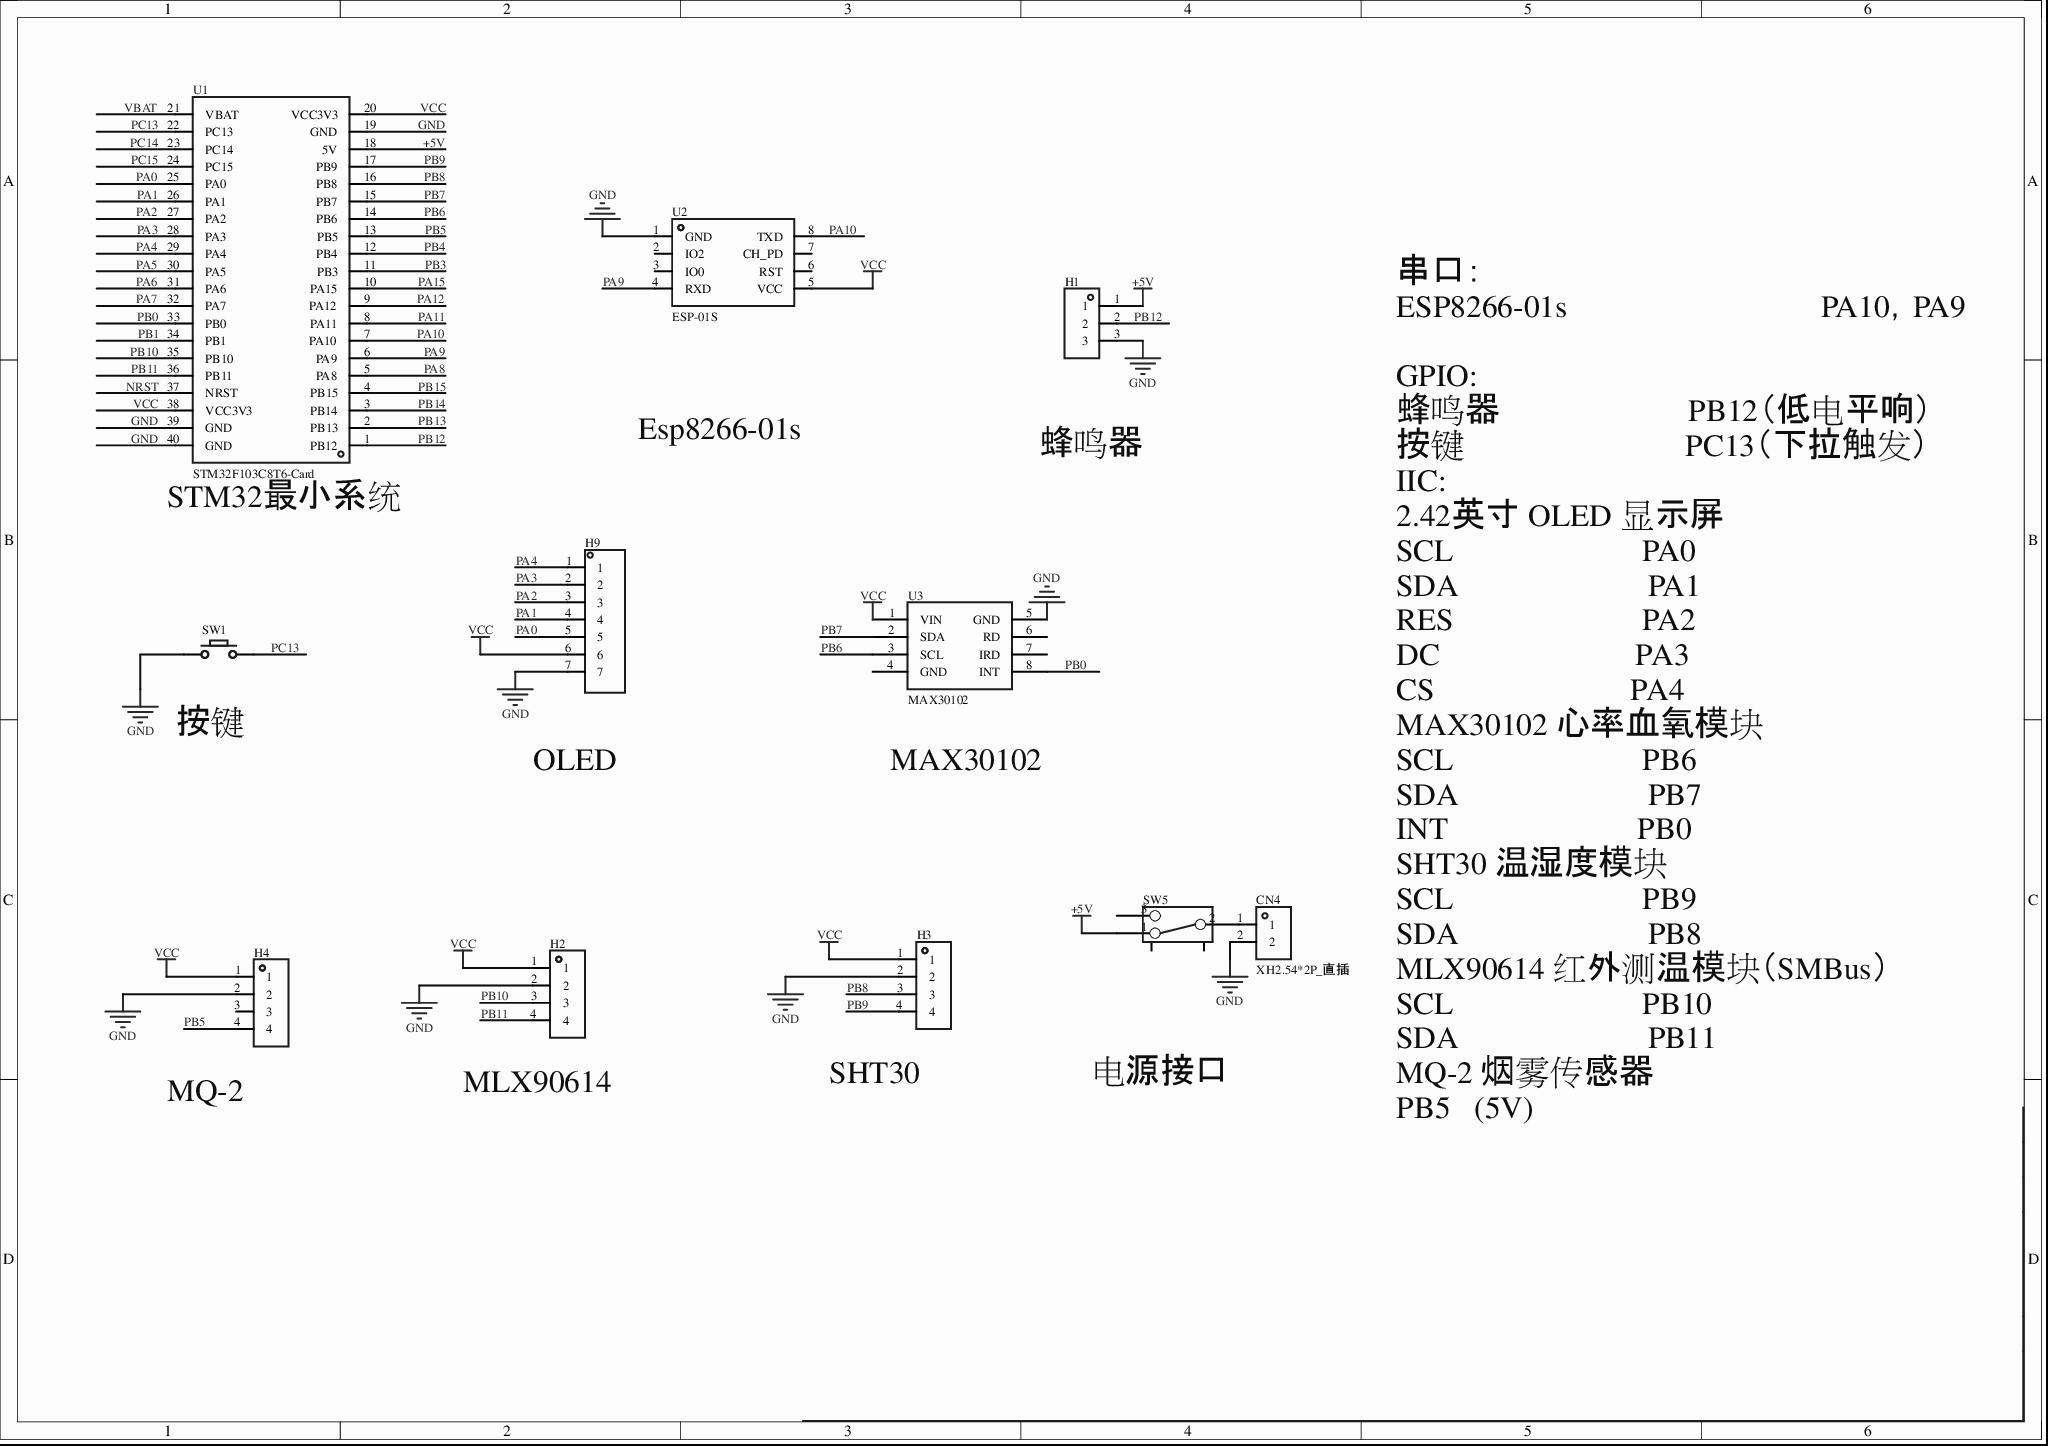
[diagram p0: MISC52061-3.schdoc]
# Altium project MISC52061-2.PrjPcb
1 sheet, 11 parts. Net scope: global (net labels, ports and power ports of the same name join across sheets).
Board file: MISC52061.pcbdoc

## Sheet MISC52061-3.schdoc
size 297 x 209 mm; Version: V1.0; @Project Name: MISC52061; @Page Count: 1; @Update Date: 2026-05-04; @Create Date: 2026-05-04; @Schematic Name: MISC52061; @Page No: 1; @Create Time: 23:22:16; @Update Time: 17:32:40; @Board Name: MISC52061

### Parts
CN4  XH2.54*2P_直插  [CONN-TH_2P-P2.50-XH2.54-2P]
H1  (no value)  [HDR-TH_3P-P2.54-V-F]
H2  (no value)  [HDR-TH_4P-P2.54-V-F]
H3  (no value)  [HDR-TH_4P-P2.54-V-F]
H4  (no value)  [HDR-TH_4P-P2.54-V-F]
H9  (no value)  [HDR-TH_7P-P2.54-V-F]
SW1  (no value)  [Key_TH_3.5x6x4.3]
SW5  (no value)  [拨动开关]
U1  STM32F103C8T6-Card  [CONN-TH_L53.3-W22.9_STM32F103C8T6-CARD]
U2  ESP-01S  [WIFIM-TH_ESP-01S]
U3  MAX30102  [MAX30102]

### Nets
+5V: H1.1 SW5.1 U1.18(5V)
GND: CN4.2 H1.3 H2.2 H3.2 H4.2 H9.7 SW1.A U1.19(GND) U1.39(GND) U1.40(GND) U2.1(GND) U3.5(GND)
VCC: H2.1 H3.1 H4.1 H9.6 U1.20(VCC3V3) U1.38(VCC3V3) U2.5(VCC) U3.1(VIN)
NRST: U1.37(NRST)
PA0: H9.5 U1.25(PA0)
PA1: H9.4 U1.26(PA1)
PA2: H9.3 U1.27(PA2)
PA3: H9.2 U1.28(PA3)
PA4: H9.1 U1.29(PA4)
PA5: U1.30(PA5)
PA6: U1.31(PA6)
PA7: U1.32(PA7)
PA8: U1.5(PA8)
PA9: U1.6(PA9) U2.4(RXD)
PA10: U1.7(PA10) U2.8(TXD)
PA11: U1.8(PA11)
PA12: U1.9(PA12)
PA15: U1.10(PA15)
PB0: U1.33(PB0) U3.8(INT)
PB1: U1.34(PB1)
PB3: U1.11(PB3)
PB4: U1.12(PB4)
PB5: H4.4 U1.13(PB5)
PB6: U1.14(PB6) U3.3(SCL)
PB7: U1.15(PB7) U3.2(SDA)
PB8: H3.3 U1.16(PB8)
PB9: H3.4 U1.17(PB9)
PB10: H2.3 U1.35(PB10)
PB11: H2.4 U1.36(PB11)
PB12: H1.2 U1.1(PB12)
PB13: U1.2(PB13)
PB14: U1.3(PB14)
PB15: U1.4(PB15)
PC13: SW1.B U1.22(PC13)
PC14: U1.23(PC14)
PC15: U1.24(PC15)
VBAT: U1.21(VBAT)
NetCN4_1: CN4.1 SW5.2

Not connected (* = marked no-connect by the designer): H4 3; SW5 3 4 5; U2 2(IO2)* 3(IO0)* 6(RST)* 7(CH_PD)*; U3 4(GND)* 6(RD)* 7(IRD)*

### Notes on the sheet
- 串口：
  ESP8266-01s  		PA10，PA9 	(串口1）
  GPIO:
  蜂鸣器      PB12（低电平响）
  按键       PC13（下拉触发）
  IIC:
  2.42英寸 OLED 显示屏
  SCL      PA0
  SDA      PA1
  RES      PA2
  DC       PA3
  CS       PA4
  MAX30102 心率血氧模块
  SCL      PB6
  SDA      PB7
  INT      PB0
  SHT30 温湿度模块
  SCL      PB9
  SDA      PB8
  MLX90614 红外测温模块（SMBus）
  SCL      PB10
  SDA      PB11
  MQ-2 烟雾传感器   
  PB5   (5V)
- (near U1) STM32最小系统
- Esp8266-01s
- 蜂鸣器
- (near SW1) 按键
- OLED
- MAX30102
- (near H4) MQ-2
- (near H2) MLX90614
- (near H3) SHT30
- 电源接口

### Library data of the parts
CN4 = XH2.54*2P_直插: 3D Model: 325c595e30db4df8abe76612dd40b0fa0819f05c4eef4c71ace90d822a990e87; 3D Model Transform: 295.275,228.346,0,180,0,0,-0.002,-20.079,-137.795; AddInBom: yes; Device: XH2.54*2P_直插; Symbol: XH2.54*2P_直插; LCSC Part Name: XH2.54*2P_直插; Supplier Part: C9900008615; Manufacturer Part: XH2.54*2P_直插; Supplier Footprint: XH2.54_2P; JLCPCB Part Class: Extended Part; Supplier: LCSC; FootprintName: CONN-TH_2P-P2.50-XH2.54-2P; ConvertToPcb: yes; ModelName: CONN-TH_2P-P2.50-XH2.54-2P
H1 = HDR-F_2.54_1x3P: Symbol: PM254V-11-03-H85; 3D Model: f3b3cc5aae9641bf9e56fc160cef875b; 3D Model Transform: 299.9994,100,0,0,0,0,0,0,-118.11; ConvertToPcb: yes; ModelName: HDR2.54-F-LI-1X3P; Device: HDR-F_2.54_1x3P; Supplier Part: C541850; Supplier Footprint: 插件; FootprintName: HDR-TH_3P-P2.54-V-F; AddInBom: yes
H2 H3 = HDR-F_2.54_1x4P: Symbol: 2.54-1*4P母; 3D Model: d187812051054f85879fcaa51a310d8e0819f05c4eef4c71ace90d822a990e87; 3D Model Transform: 419.6842,98.464,0,0,0,0,0,0,-118.11; ConvertToPcb: yes; Device: HDR-F_2.54_1x4P; Supplier Part: C2718488; Supplier Footprint: 插件; FootprintName: HDR-TH_4P-P2.54-V-F; AddInBom: yes; ModelName: HDR-TH_4P-P2.54-V-F
H4 = HDR-F_2.54_1x4P: Symbol: 2.54-1*4P母; ConvertToPcb: yes; ModelId: d187812051054f85879fcaa51a310d8e0819f05c4eef4c71ace90d822a990e87; ModelTransform: 419.6842,98.464,0,0,0,0,0,0,-118.11; Device: HDR-F_2.54_1x4P; FootprintName: HDR-TH_4P-P2.54-V-F; AddInBom: yes; SupplierPart: C2718488; Supplier Footprint: 插件; ModelName: HDR-TH_4P-P2.54-V-F
H9 = HDR-F_2.54_1x7P: Symbol: 220S-1*7P H=8.5MM Ytype Gold-plated; ConvertToPcb: yes; ModelId: 4c31987253bc43b9b52c17be2a6d3f910819f05c4eef4c71ace90d822a990e87; ModelName: HDR-TH_7P-P2.54-F-LI-1X7P; ModelTransform: 715.7466,94.488,0,0,0,0,0,0,-118.11; Device: HDR-F_2.54_1x7P; AddInBom: yes; SupplierPart: C124418; Supplier Footprint: 插件; FootprintName: HDR-TH_7P-P2.54-V-F
SW1 = Key_TH_3.5x6x4.3: ConvertToPcb: yes; ModelId: c3523f9014d949d7ba5445190a3178990819f05c4eef4c71ace90d822a990e87; ModelName: SW-TH_L6.0-W3.5-H5.0-P6.5; ModelTransform: 308.49,137.8,335.08,0,0,0,0,0,-129.92; Symbol: Key_TH_3.5x6x4.3; Device: Key_TH_3.5x6x4.3; AddInBom: yes; Supplier Footprint: 插件; FootprintName: Key_TH_3.5x6x4.3
SW5 = 拨动开关_正: ConvertToPcb: yes; ModelId: 4321fe59a4074cbfb4989553f297c68f0819f05c4eef4c71ace90d822a990e87; ModelName: SW-TH_SS-12D02-VG4; ModelTransform: 370.09,208.7,472.35,0,0,0,0,0,-110; Device: 拨动开关_正; Symbol: 拨动开关; FootprintName: 拨动开关; AddInBom: yes; Supplier Footprint: 插件
U1 = STM32F103C8T6-Card: AddInBom: yes; Device: STM32F103C8T6-Card; Symbol: STM32F103C8T6-CARD; FootprintName: CONN-TH_L53.3-W22.9_STM32F103C8T6-CARD; LCSC Part Name: STM32F103C8T6-Card; SupplierPart: C9900077949; ManufacturerPart: STM32F103C8T6-Card; Supplier Footprint: 插件; Supplier: LCSC; ConvertToPcb: yes
U2 = ESP-01S_C111009: 3D Model: eb7175da78ae48b3b1568cfe3027405f0819f05c4eef4c71ace90d822a990e87; 3D Model Transform: 582.676,976.37608,0,0,0,0,0,388.346,-118.11; AddInBom: yes; Symbol: ESP-01S; Device: ESP-01S_C111009; LCSC Part Name: ESP-01S; Supplier Part: C111009; Manufacturer Part: ESP-01S; Supplier Footprint: -; JLCPCB Part Class: Extended Part; Supplier: LCSC; ConvertToPcb: yes; FootprintName: WIFIM-TH_ESP-01S; ModelName: WIFIM-TH_ESP-01S
U3 = MAX30102: AddInBom: yes; Symbol: MAX30102; Device: MAX30102; ConvertToPcb: yes; FootprintName: MAX30102